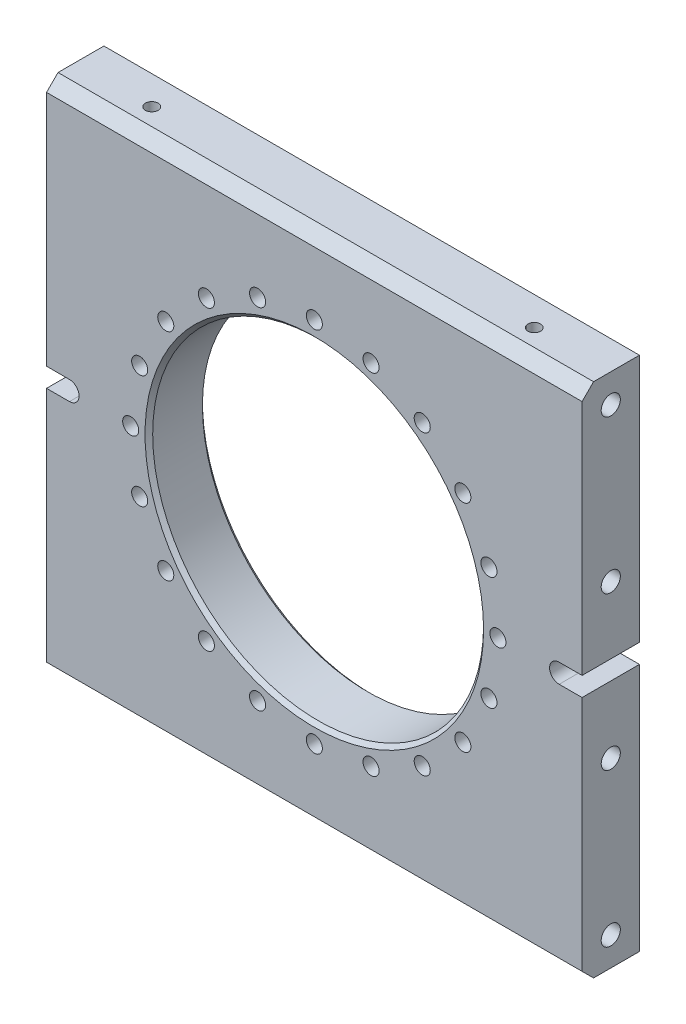
from build123d import *

# Parameters (mm, degrees)
SKETCH_1_W                  = 140
SKETCH_1_H                  = 135
SKETCH_1_R                  = 43.25
EXTRUDE_1_DEPTH             = 7.5
HOLE_WIZARD_M6_1_AT_2_COUNT = 2
HOLE_WIZARD_M6_1_AT_2_PITCH = 40
HOLE_WIZARD_M6_1_AT_3_COUNT = 2
HOLE_WIZARD_M6_1_AT_3_PITCH = 80
HOLE_WIZARD_M6_1_AT_4_COUNT = 2
HOLE_WIZARD_M6_1_AT_4_PITCH = 40
HOLE_WIZARD_M5_1_D          = 4.2
CHAMFER_1_SIZE              = 1
PATTERN_CIRCULAR_1_COUNT    = 20
CUT_EXTRUDE_1_DEPTH         = 99.393343271
HOLE_WIZARD_M4_1_AT_2_COUNT = 2
HOLE_WIZARD_M4_1_AT_2_PITCH = 100
CHAMFER_2_SIZE              = 3


with BuildPart() as part:
    # 草图1 → 凸台-拉伸1 (new, symmetric)
    with BuildSketch(Plane.XY):
        Rectangle(SKETCH_1_W, SKETCH_1_H)
        Circle(SKETCH_1_R, mode=Mode.SUBTRACT)
    extrude(amount=EXTRUDE_1_DEPTH, both=True)

    # 草图3 → M6 螺纹孔1 (revolve, cut)
    with BuildSketch(Plane(origin=(70, -20, 0), x_dir=(0, 0, -1), z_dir=(0, 1, 0))):
        Polygon((0, 0), (0, 19.502151548), (2.5, 18), (2.5, 0), align=None)
    hole_wizard_m6_1 = revolve(axis=Axis((76.35, -20, 0), (-1, 0, 0)), mode=Mode.SUBTRACT)

    # M6 螺纹孔1 at 2: M6 螺纹孔1 ×2
    with Locations(*[(0, -i * HOLE_WIZARD_M6_1_AT_2_PITCH, 0) for i in range(1, HOLE_WIZARD_M6_1_AT_2_COUNT)]):
        add(hole_wizard_m6_1, mode=Mode.SUBTRACT)

    # M6 螺纹孔1 at 3: M6 螺纹孔1 ×2
    with Locations(*[(0, i * HOLE_WIZARD_M6_1_AT_3_PITCH, 0) for i in range(1, HOLE_WIZARD_M6_1_AT_3_COUNT)]):
        add(hole_wizard_m6_1, mode=Mode.SUBTRACT)

    # M6 螺纹孔1 at 4: M6 螺纹孔1 ×2
    with Locations(*[(0, i * HOLE_WIZARD_M6_1_AT_4_PITCH, 0) for i in range(1, HOLE_WIZARD_M6_1_AT_4_COUNT)]):
        add(hole_wizard_m6_1, mode=Mode.SUBTRACT)

    # 镜向2: M6 螺纹孔1 across plane
    add(hole_wizard_m6_1.mirror(Plane(origin=(0, 0, 0), x_dir=(0, 0, 1), z_dir=(1, 0, 0))), mode=Mode.SUBTRACT)

    # 镜向2 copy 1 sketch → 镜向2 copy 1 (revolve, cut)
    with BuildSketch(Plane(origin=(-70, -60, 0), x_dir=(0, 0, -1), z_dir=(0, 1, 0))):
        Polygon((0, 0), (0, -19.502151548), (2.5, -18), (2.5, 0), align=None)
    revolve(axis=Axis((-76.35, -60, 0), (-1, 0, 0)), mode=Mode.SUBTRACT)

    # 镜向2 copy 2 sketch → 镜向2 copy 2 (revolve, cut)
    with BuildSketch(Plane(origin=(-70, 60, 0), x_dir=(0, 0, -1), z_dir=(0, 1, 0))):
        Polygon((0, 0), (0, -19.502151548), (2.5, -18), (2.5, 0), align=None)
    revolve(axis=Axis((-76.35, 60, 0), (-1, 0, 0)), mode=Mode.SUBTRACT)

    # 镜向2 copy 3 sketch → 镜向2 copy 3 (revolve, cut)
    with BuildSketch(Plane(origin=(-70, 20, 0), x_dir=(0, 0, -1), z_dir=(0, 1, 0))):
        Polygon((0, 0), (0, -19.502151548), (2.5, -18), (2.5, 0), align=None)
    revolve(axis=Axis((-76.35, 20, 0), (-1, 0, 0)), mode=Mode.SUBTRACT)

    # M5 螺纹孔1 (through all)
    with Locations(Plane.XY.offset(7.5)):
        with Locations((0, 48)):
            hole_wizard_m5_1 = Hole(HOLE_WIZARD_M5_1_D / 2)

    # 倒角1
    chamfer_1_edges = [part.edges().sort_by_distance(p)[0] for p in [
        (-43.25, 0, -7.5),
        (-43.25, 0, 7.5),
    ]]
    chamfer(chamfer_1_edges, length=CHAMFER_1_SIZE)

    # 阵列(圆周)1: M5 螺纹孔1 ×20 about axis
    pattern_circular_1_axis = Axis((0, 0, 0), (0, 0, 1))
    for i in range(1, PATTERN_CIRCULAR_1_COUNT):
        add(hole_wizard_m5_1.rotate(pattern_circular_1_axis, i * 360 / PATTERN_CIRCULAR_1_COUNT), mode=Mode.SUBTRACT)

    # 草图6 → 切除-拉伸1 (cut, through all)
    with BuildSketch(Plane.XY.offset(7.5)):
        with BuildLine():
            Line((70, 2.5), (64, 2.5))
            ThreePointArc((64, 2.5), (61.5, 0), (64, -2.5))
            Line((64, -2.5), (70, -2.5))
            Line((70, -2.5), (70, 2.5))
        make_face()
        with BuildLine():
            Line((-70, -2.5), (-64, -2.5))
            ThreePointArc((-64, -2.5), (-61.5, 0), (-64, 2.5))
            Line((-64, 2.5), (-70, 2.5))
            Line((-70, 2.5), (-70, -2.5))
        make_face()
    extrude(amount=-CUT_EXTRUDE_1_DEPTH, mode=Mode.SUBTRACT)

    # 草图8 → M4 螺纹孔1 (revolve, cut)
    with BuildSketch(Plane(origin=(-50, -67.5, 0), x_dir=(0, 0, -1), z_dir=(1, 0, 0))):
        Polygon((0, 0), (0, 18.091420021), (1.65, 17.1), (1.65, 0), align=None)
    hole_wizard_m4_1 = revolve(axis=Axis((-50, -73.85, 0), (0, 1, 0)), mode=Mode.SUBTRACT)

    # M4 螺纹孔1 at 2: M4 螺纹孔1 ×2
    with Locations(*[(i * HOLE_WIZARD_M4_1_AT_2_PITCH, 0, 0) for i in range(1, HOLE_WIZARD_M4_1_AT_2_COUNT)]):
        add(hole_wizard_m4_1, mode=Mode.SUBTRACT)

    # 镜向3: M4 螺纹孔1 across plane
    add(hole_wizard_m4_1.mirror(Plane.ZX), mode=Mode.SUBTRACT)

    # 镜向3 copy 1 sketch → 镜向3 copy 1 (revolve, cut)
    with BuildSketch(Plane(origin=(50, 67.5, 0), x_dir=(0, 0, -1), z_dir=(1, 0, 0))):
        Polygon((0, 0), (0, -18.091420021), (1.65, -17.1), (1.65, 0), align=None)
    revolve(axis=Axis((50, 73.85, 0), (0, 1, 0)), mode=Mode.SUBTRACT)

    # 倒角2
    chamfer_2_edges = [part.edges().sort_by_distance(p)[0] for p in [
        (0, 67.5, 7.5),
        (0, -67.5, 7.5),
    ]]
    chamfer(chamfer_2_edges, length=CHAMFER_2_SIZE)


solid = part.part
